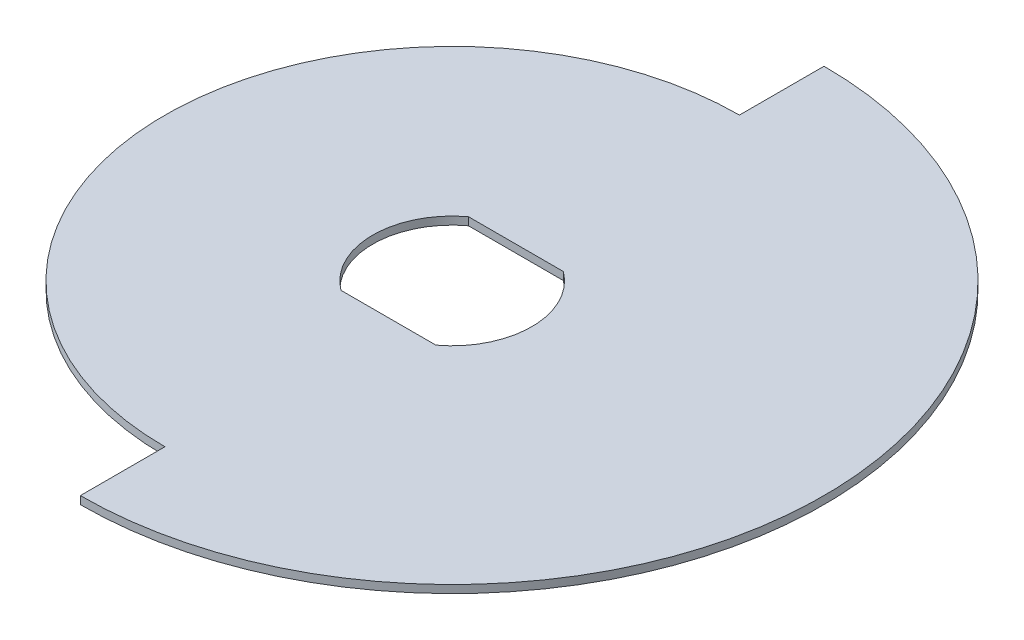
SolidWorks part; units mm, degrees
material "普通碳钢"
ref_plane "Front Plane" through (0, 0, 0) normal (0, 0, 1) x (1, 0, 0)
ref_plane "Top Plane" through (0, 0, 0) normal (0, 1, 0) x (1, 0, 0)
ref_plane "Right Plane" through (0, 0, 0) normal (1, 0, 0) x (0, 0, -1)
sketch "Sketch1" plane through (0, 0, 0) normal (0, 1, 0) x (1, 0, 0)
  circle A0 centre (0, 0) radius 10.1
  circle A1 centre (0, 0) radius 47.25
  dimension "D1" = 20.2
  dimension "D2" = 94.5
extrude "Boss-Extrude1" add sketch "Sketch1" along normal blind 1
sketch "Sketch2" plane through (0, 0, 0) normal (0, -1, 0) x (1, 0, 0)
  line L1 (6.0332, -8.1) -> (-6.0332, -8.1)
  line L3 (6.0332, 8.1) -> (-6.0332, 8.1)
  arc A0 (-6.0332, -8.1) -> (6.0332, -8.1) centre (0, 0) ccw
  arc A1 (6.0332, 8.1) -> (-6.0332, 8.1) centre (0, 0) ccw
  point P0 (0, 0)
  dimension "D2" = 20.2
  dimension "D1" = 8.1
  dimension "D3" = 8.1
extrude "Boss-Extrude2" add sketch "Sketch2" against normal blind 1
sketch "Sketch3" plane through (0, 0, 0) normal (0, -1, 0) x (1, 0, 0)
  line L0 (0, 47.25) -> (0, 36.5)
  line L1 (0, -36.5) -> (0, -47.25)
  arc A0 (0, 36.5) -> (0, -36.5) centre (0, 0) ccw
  circle A2 centre (0, 0) radius 47.25 construction
  arc A3 (0, 47.25) -> (0, -47.25) centre (0, 0) ccw
  dimension "D1" = 73
extrude "Cut-Extrude1" cut sketch "Sketch3" against normal blind 10
